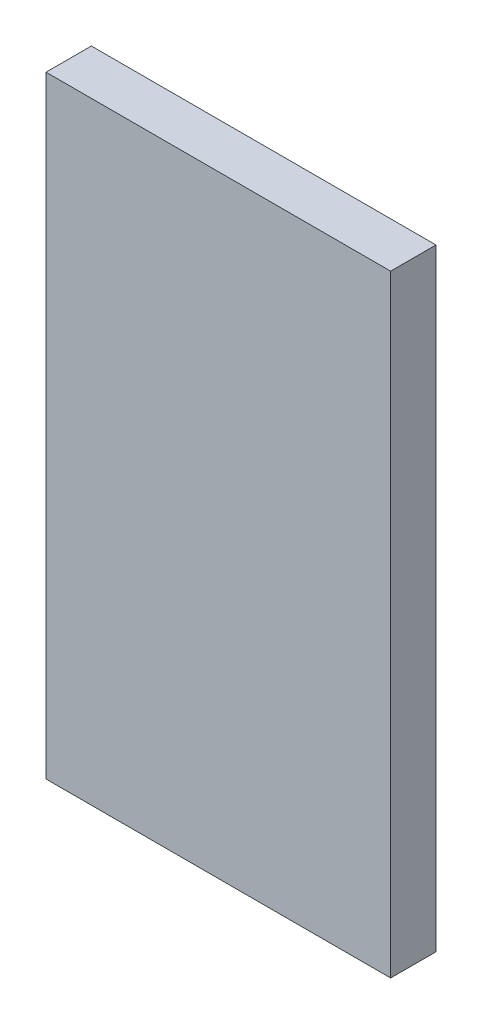
from build123d import *

# Parameters (mm, degrees)
SKETCH1_W           = 152
SKETCH1_H           = 270
BOSS_EXTRUDE1_DEPTH = 20


with BuildPart() as part:
    # Sketch1 → Boss-Extrude1 (new body)
    with BuildSketch(Plane.XY):
        with Locations((76, 135)):
            Rectangle(SKETCH1_W, SKETCH1_H)
    extrude(amount=BOSS_EXTRUDE1_DEPTH)


solid = part.part
